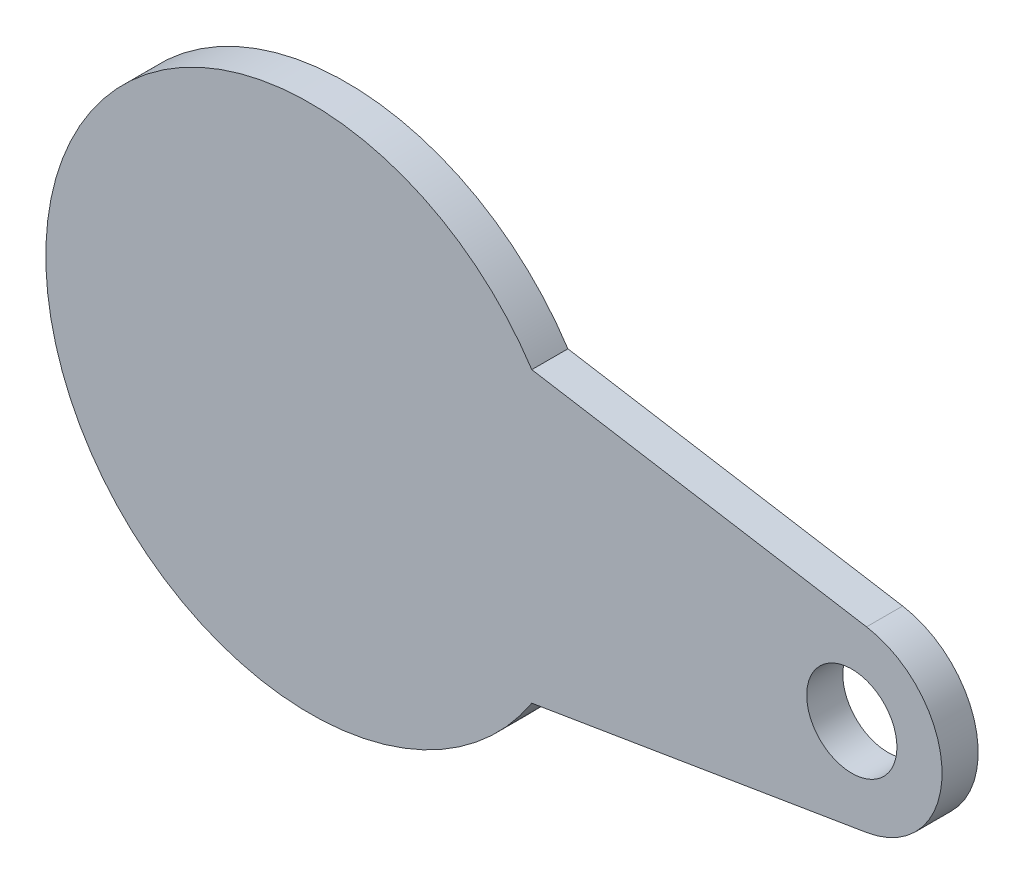
SolidWorks part; units mm, degrees
ref_plane "Front Plane" through (0, 0, 0) normal (0, 0, 1) x (1, 0, 0)
ref_plane "Top Plane" through (0, 0, 0) normal (0, 1, 0) x (1, 0, 0)
ref_plane "Right Plane" through (0, 0, 0) normal (1, 0, 0) x (0, 0, -1)
other "Configuration Table"
sketch "Sketch1" plane through (0, 0, 0) normal (0, 0, 1) x (1, 0, 0)
  line L0 (122.7284, 80) -> (308.1591, 49.3298)
  line L1 (0, 0) -> (300, 0) construction
  line L2 (122.7284, -80) -> (308.1591, -49.3298)
  arc A0 (122.7284, 80) -> (122.7284, -80) centre (0, 0) ccw
  arc A1 (308.1591, -49.3298) -> (308.1591, 49.3298) centre (300, 0) ccw
  circle A2 centre (300, 0) radius 25
  dimension "D1" = 293
  dimension "D2" = 100
  dimension "D3" = 300
  dimension "D4" = 50
  dimension "D5" = 160
  dimension "D6" = 80
extrude "Boss-Extrude1" add sketch "Sketch1" along normal blind 20
